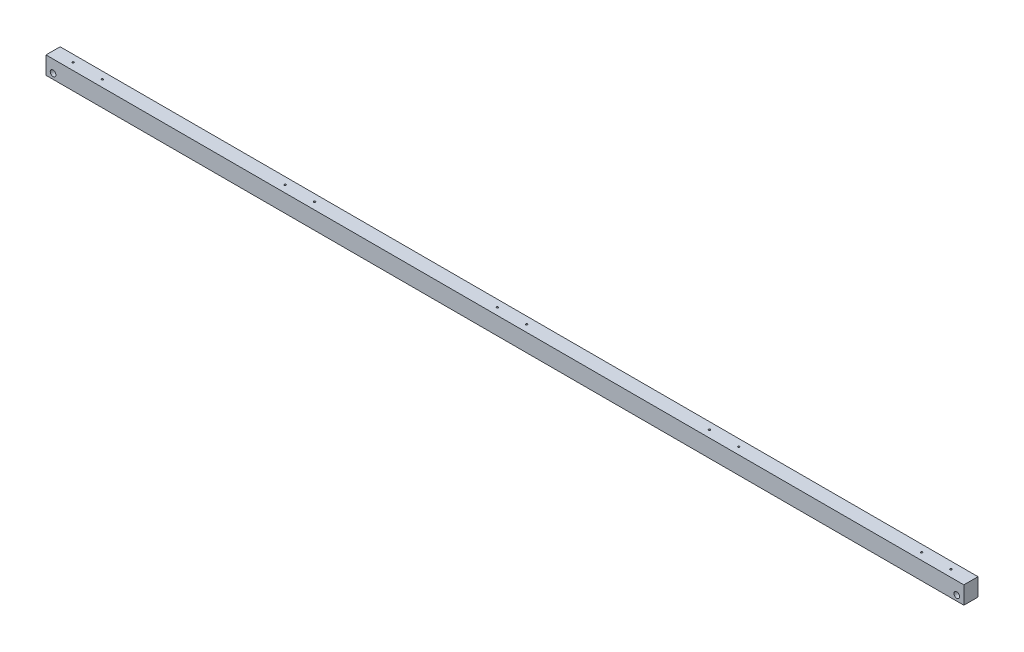
from build123d import *

# Parameters (mm, degrees)
SKETCH1_W           = 2596
SKETCH1_H           = 40
BOSS_EXTRUDE1_DEPTH = 50
SKETCH2_R           = 2.5
CUT_EXTRUDE1_DEPTH  = 50
SKETCH3_R           = 8
CUT_EXTRUDE2_DEPTH  = 50


with BuildPart() as part:
    # Sketch1 → Boss-Extrude1 (new body)
    with BuildSketch(Plane(origin=(0, 0, 0), x_dir=(1, 0, 0), z_dir=(0, 1, 0))):
        Rectangle(SKETCH1_W, SKETCH1_H)
    extrude(amount=BOSS_EXTRUDE1_DEPTH)

    # Sketch2 → Cut-Extrude1 (cut)
    with BuildSketch(Plane.XZ):
        with Locations(Location((1241.5, 0, 0), (0, 0, 270))):
            Circle(SKETCH2_R)
        with Locations(Location((1158.5, 0, 0), (0, 0, 270))):
            Circle(SKETCH2_R)
        with Locations(Location((641.5, 0, 0), (0, 0, 270))):
            Circle(SKETCH2_R)
        with Locations(Location((558.5, 0, 0), (0, 0, 270))):
            Circle(SKETCH2_R)
        with Locations(Location((41.5, 0, 0), (0, 0, 270))):
            Circle(SKETCH2_R)
        with Locations(Location((-41.5, 0, 0), (0, 0, 90))):
            Circle(SKETCH2_R)
        with Locations(Location((-558.5, 0, 0), (0, 0, 90))):
            Circle(SKETCH2_R)
        with Locations(Location((-641.5, 0, 0), (0, 0, 90))):
            Circle(SKETCH2_R)
        with Locations(Location((-1158.5, 0, 0), (0, 0, 90))):
            Circle(SKETCH2_R)
        with Locations(Location((-1241.5, 0, 0), (0, 0, 90))):
            Circle(SKETCH2_R)
    extrude(amount=-CUT_EXTRUDE1_DEPTH, mode=Mode.SUBTRACT)

    # Sketch3 → Cut-Extrude2 (cut)
    with BuildSketch(Plane(origin=(0, 0, -20), x_dir=(-1, 0, 0), z_dir=(0, 0, -1))):
        with Locations((-1278, 15)):
            Circle(SKETCH3_R)
        with Locations((1278, 15)):
            Circle(SKETCH3_R)
    extrude(amount=-CUT_EXTRUDE2_DEPTH, mode=Mode.SUBTRACT)


solid = part.part
